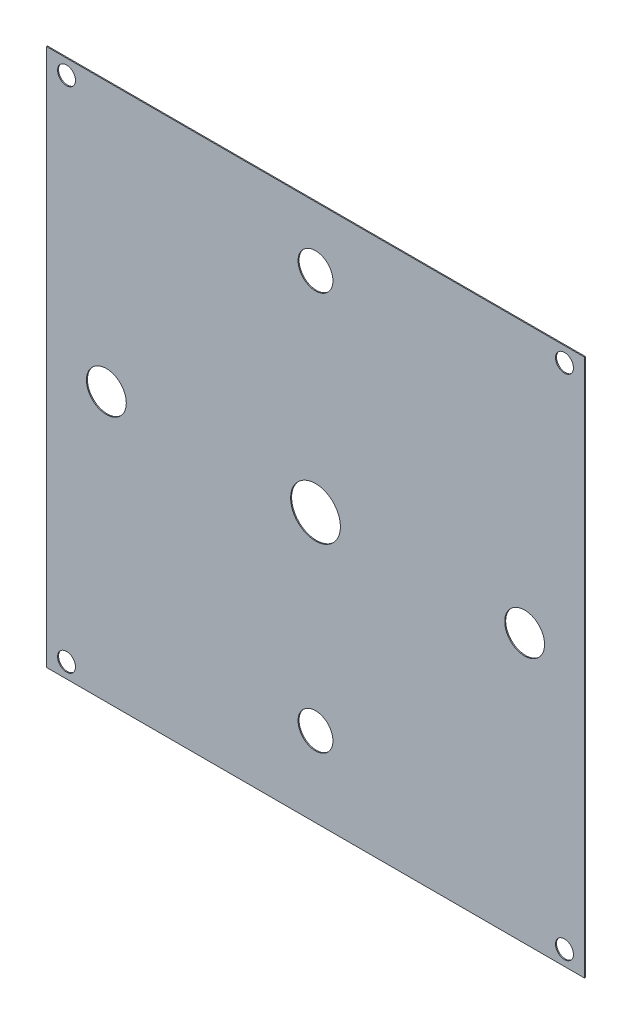
from build123d import *

# Parameters (mm, degrees)
SKETCH_1_W          = 540
SKETCH_1_H          = 540
EXTRUDE_1_DEPTH     = 1
SKETCH_2_R          = 9
CUT_EXTRUDE_1_DEPTH = 382.838971295
SKETCH_3_R          = 20
CUT_EXTRUDE_2_DEPTH = 382.838971295
SKETCH_4_R          = 25
CUT_EXTRUDE_3_DEPTH = 10
SKETCH_5_R          = 17.5
CUT_EXTRUDE_4_DEPTH = 382.838971295


with BuildPart() as part:
    # 草图1 → 凸台-拉伸1 (new body)
    with BuildSketch(Plane.XY):
        Rectangle(SKETCH_1_W, SKETCH_1_H)
    extrude(amount=EXTRUDE_1_DEPTH)

    # 草图2 → 切除-拉伸1 (cut, through all)
    with BuildSketch(Plane(origin=(0, 0, 0), x_dir=(-1, 0, 0), z_dir=(0, 0, -1))):
        with Locations((250, -255)):
            Circle(SKETCH_2_R)
        with Locations((-250, -255)):
            Circle(SKETCH_2_R)
        with Locations((250, 255)):
            Circle(SKETCH_2_R)
        with Locations((-250, 255)):
            Circle(SKETCH_2_R)
    extrude(amount=-CUT_EXTRUDE_1_DEPTH, mode=Mode.SUBTRACT)

    # 草图3 → 切除-拉伸2 (cut, through all)
    with BuildSketch(Plane.XY.offset(1)):
        with Locations((-210, 0)):
            Circle(SKETCH_3_R)
        with Locations((210, 0)):
            Circle(SKETCH_3_R)
    extrude(amount=-CUT_EXTRUDE_2_DEPTH, mode=Mode.SUBTRACT)

    # 草图4 → 切除-拉伸3 (cut)
    with BuildSketch(Plane.XY.offset(1)):
        Circle(SKETCH_4_R)
    extrude(amount=-CUT_EXTRUDE_3_DEPTH, mode=Mode.SUBTRACT)

    # 草图5 → 切除-拉伸4 (cut, through all)
    with BuildSketch(Plane(origin=(0, 0, 0), x_dir=(-1, 0, 0), z_dir=(0, 0, -1))):
        with Locations((0, -190)):
            Circle(SKETCH_5_R)
        with Locations((0, 210)):
            Circle(SKETCH_5_R)
    extrude(amount=-CUT_EXTRUDE_4_DEPTH, mode=Mode.SUBTRACT)


solid = part.part
